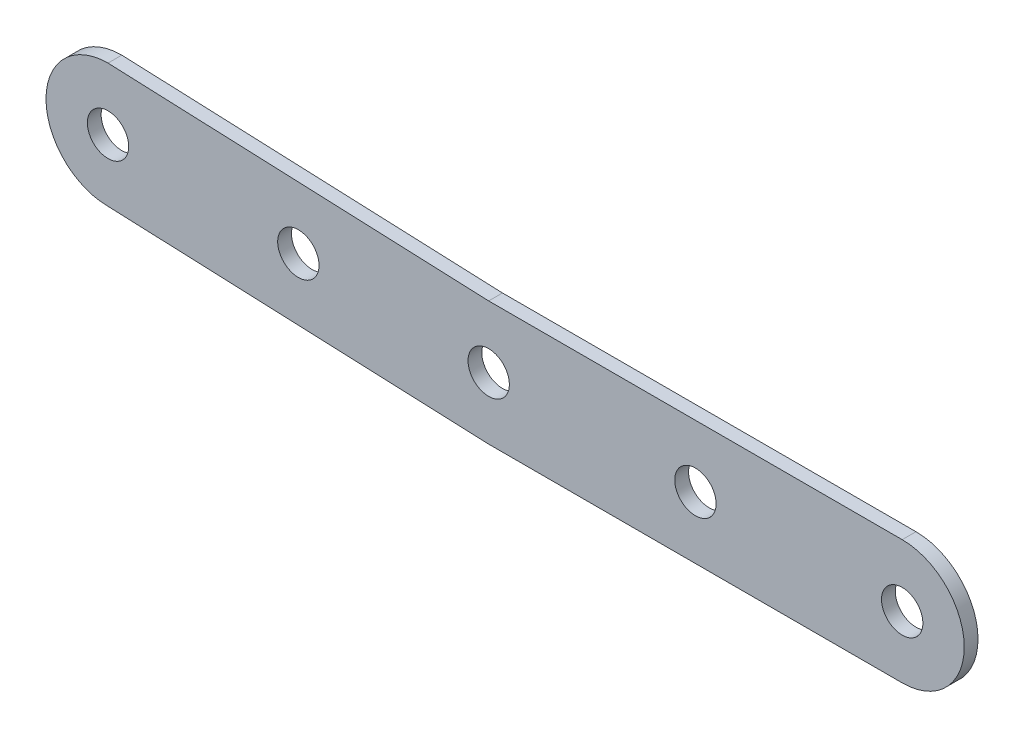
SolidWorks part; units mm, degrees
ref_plane "Front Plane" through (0, 0, 0) normal (0, 0, 1) x (1, 0, 0)
ref_plane "Top Plane" through (0, 0, 0) normal (0, 1, 0) x (1, 0, 0)
ref_plane "Right Plane" through (0, 0, 0) normal (1, 0, 0) x (0, 0, -1)
other "Configuration Table"
sketch "Sketch1" plane through (0, 0, 0) normal (0, 0, 1) x (1, 0, 0)
  line L0 (0, 0) -> (55.2341, -2.2715) construction
  line L1 (55.2341, -2.2715) -> (115.2341, -2.2715) construction
  line L2 (0, 9) -> (55.2341, 6.7285)
  line L3 (55.2341, 6.7285) -> (115.2341, 6.7285)
  line L5 (0, -9) -> (55.2341, -11.2715)
  line L6 (55.2341, -11.2715) -> (115.2341, -11.2715)
  arc A0 (0, 9) -> (0, -9) centre (0, 0) ccw
  arc A1 (115.2341, -11.2715) -> (115.2341, 6.7285) centre (115.2341, -2.2715) ccw
  circle A2 centre (0, 0) radius 3
  circle A3 centre (55.2341, -2.2715) radius 3
  circle A4 centre (115.2341, -2.2715) radius 3
  circle A5 centre (27.617, -1.1357) radius 3
  circle A6 centre (85.2341, -2.2715) radius 3
  dimension "D4" = 18
  dimension "D5" = 6
  dimension "D1" = 2.2715
  dimension "D2" = 115.2341
  dimension "D3" = 177.645
extrude "Boss-Extrude1" add sketch "Sketch1" along normal blind 2
